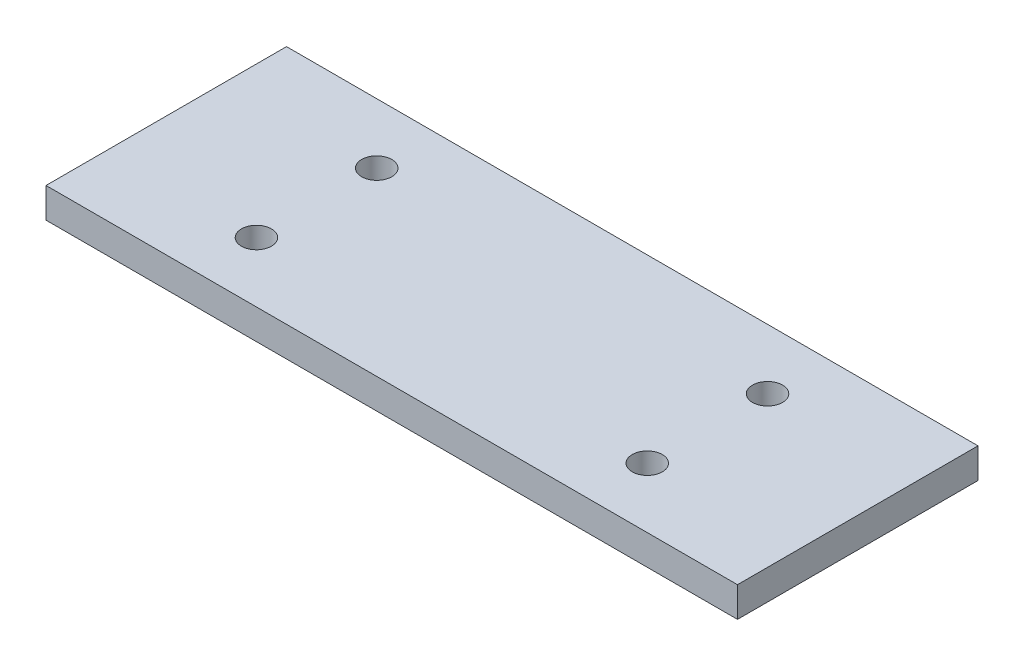
from build123d import *

# Parameters (mm, degrees)
SKETCH1_W           = 115
SKETCH1_H           = 5
BOSS_EXTRUDE1_DEPTH = 40
SKETCH2_R           = 2.5
CUT_EXTRUDE1_DEPTH  = 40


with BuildPart() as part:
    # Sketch1 → Boss-Extrude1 (new body)
    with BuildSketch(Plane.XY):
        Rectangle(SKETCH1_W, SKETCH1_H)
    extrude(amount=-BOSS_EXTRUDE1_DEPTH)

    # Sketch2 → Cut-Extrude1 (cut)
    with BuildSketch(Plane(origin=(0, 2.5, 0), x_dir=(1, 0, 0), z_dir=(0, 1, 0))):
        with Locations(Location((-32.5, 30, 0), (0, 0, 270))):
            Circle(SKETCH2_R)
        with Locations(Location((32.5, 30, 0), (0, 0, 270))):
            Circle(SKETCH2_R)
        with Locations(Location((-32.5, 10, 0), (0, 0, 270))):
            Circle(SKETCH2_R)
        with Locations(Location((32.5, 10, 0), (0, 0, 270))):
            Circle(SKETCH2_R)
    extrude(amount=-CUT_EXTRUDE1_DEPTH, mode=Mode.SUBTRACT)


solid = part.part
